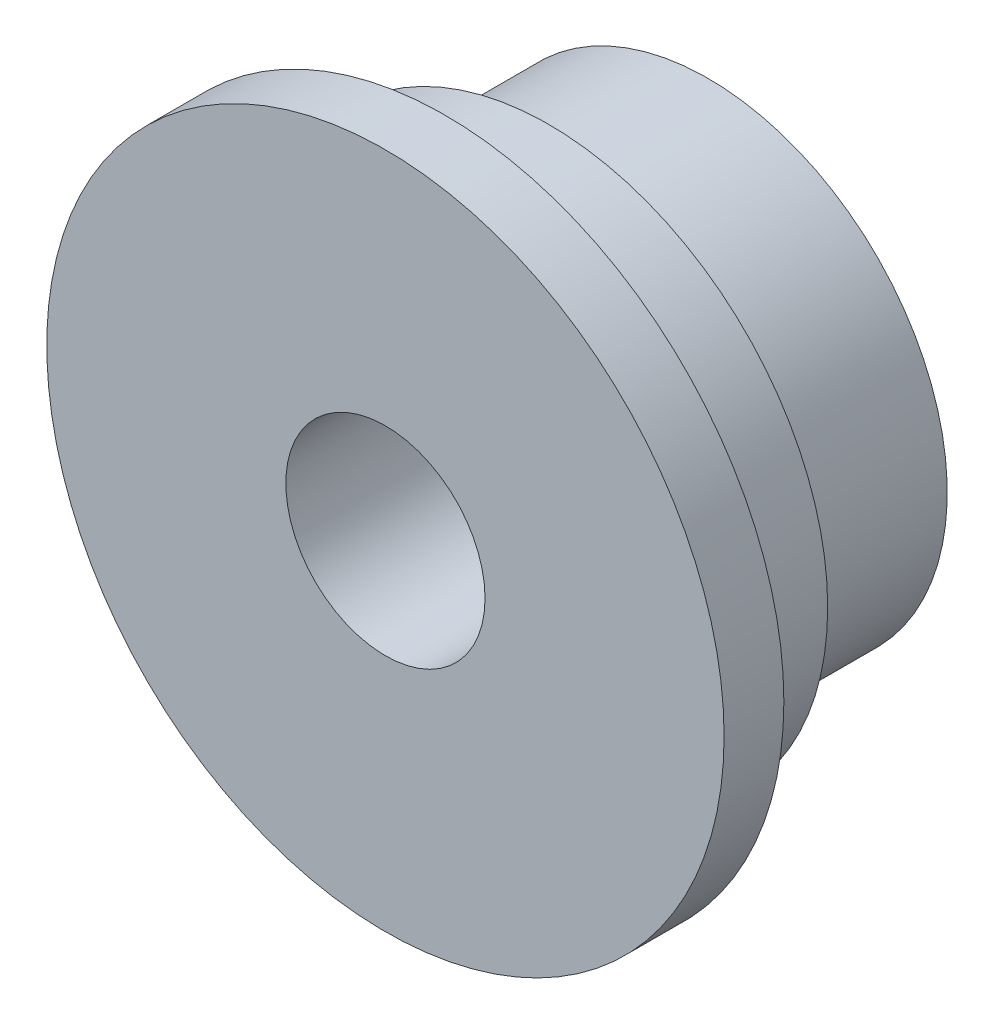
from build123d import *

# Parameters (mm, degrees)
SKETCH1_R               = 70
BOSS_EXTRUDE1_DEPTH     = 26
SKETCH2_R               = 85
BOSS_EXTRUDE2_DEPTH     = 15
SKETCH3_R               = 60
BOSS_EXTRUDE3_DEPTH     = 40
CUT_EXTRUDE1_DEPTH      = 145.951716099
CUT_EXTRUDE1_DEPTH_BACK = 145.951716099
SKETCH4_R               = 25


with BuildPart() as part:
    # Sketch1 → Boss-Extrude1 (new body)
    with BuildSketch(Plane.XY):
        Circle(SKETCH1_R)
    extrude(amount=BOSS_EXTRUDE1_DEPTH)

    # Sketch2 → Boss-Extrude2 (add)
    with BuildSketch(Plane.XY.offset(26)):
        Circle(SKETCH2_R)
    extrude(amount=BOSS_EXTRUDE2_DEPTH)

    # Sketch3 → Boss-Extrude3 (add)
    with BuildSketch(Plane(origin=(0, 0, 0), x_dir=(-1, 0, 0), z_dir=(0, 0, -1))):
        Circle(SKETCH3_R)
    extrude(amount=BOSS_EXTRUDE3_DEPTH)

    # Sketch4 → Cut-Extrude1 (cut, two sides: drawn at the far end of the back side and taken through both)
    with BuildSketch(Plane.XY.offset(41).offset(-CUT_EXTRUDE1_DEPTH_BACK)):
        Circle(SKETCH4_R)
    extrude(amount=CUT_EXTRUDE1_DEPTH + CUT_EXTRUDE1_DEPTH_BACK, mode=Mode.SUBTRACT)


solid = part.part
